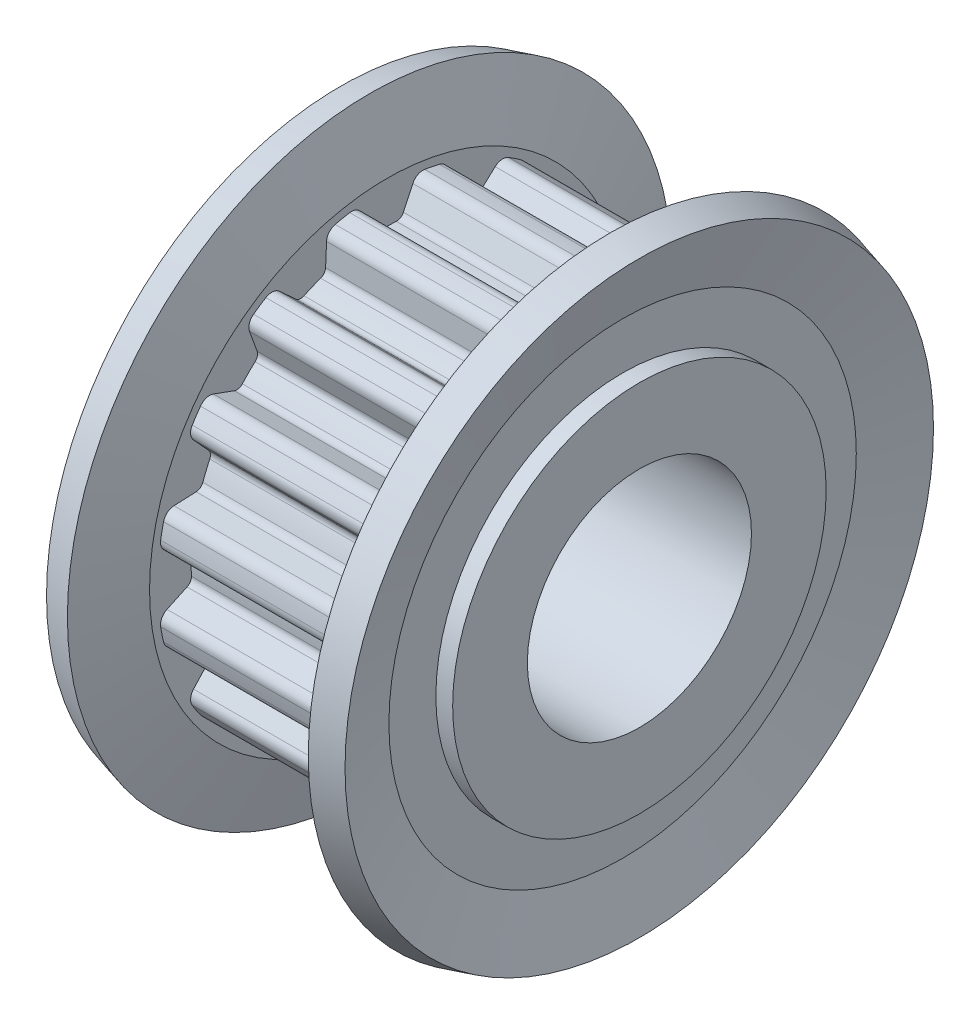
from build123d import *

# Parameters (mm, degrees)
SKETCH_2_W          = 64
SKETCH_2_H          = 64
CUT_EXTRUDE_1_DEPTH = 11


with BuildPart() as part:
    # 草图1 → 旋转1 (revolve)
    with BuildSketch(Plane.XY, mode=Mode.PRIVATE) as revolve_1_sk:
        Polygon((0, 9.8), (0, 6.2), (0.2, 6), (16, 6), (16, 10), (15.1, 10), (15.1, 12.513835473), (15.991930053, 15.754514664), (14.449291918, 16.179093968), (13.5, 12.73), (2.5, 12.73), (1.550708082, 16.179093968), (0.008069947, 15.754514664), (0.9, 12.513835473), (0.9, 10), (0.2, 10), align=None)
    revolve(revolve_1_sk.sketch.rotate(Axis((28, 0, 0), (-1, 0, 0)), 270), axis=Axis((28, 0, 0), (-1, 0, 0)))

    # 草图2 → 切除-拉伸1 (cut)
    with BuildSketch(Plane(origin=(2.5, 0, 0), x_dir=(0, 0, -1), z_dir=(1, 0, 0))):
        Rectangle(SKETCH_2_W, SKETCH_2_H)
        with BuildLine():
            Line((-11.421675295, -3.251314352), (-10.234355553, -3.303153851))
            ThreePointArc((-10.234355553, -3.303153851), (-10.014882256, -3.380486909), (-9.875590343, -3.566891557))
            ThreePointArc((-9.875590343, -3.566891557), (-9.700735091, -4.01817604), (-9.505270107, -4.460923692))
            ThreePointArc((-9.505270107, -4.460923692), (-9.471956373, -4.691225939), (-9.5724647, -4.901099725))
            Line((-9.5724647, -4.901099725), (-10.37537048, -5.777317628))
            ThreePointArc((-10.37537048, -5.777317628), (-10.530438739, -6.127247702), (-10.442388892, -6.499731859))
            ThreePointArc((-10.442388892, -6.499731859), (-10.336079998, -6.667492053), (-10.227076231, -6.833513866))
            ThreePointArc((-10.227076231, -6.833513866), (-10.115406006, -6.997754021), (-10.001098443, -7.160169686))
            ThreePointArc((-10.001098443, -7.160169686), (-9.690663174, -7.38406064), (-9.308027896, -7.374708689))
            Line((-9.308027896, -7.374708689), (-8.191249371, -6.968234547))
            ThreePointArc((-8.191249371, -6.968234547), (-7.958888404, -6.955692181), (-7.758865485, -7.074602913))
            ThreePointArc((-7.758865485, -7.074602913), (-7.424621202, -7.424621202), (-7.074602913, -7.758865485))
            ThreePointArc((-7.074602913, -7.758865485), (-6.955692181, -7.958888404), (-6.968234547, -8.191249371))
            Line((-6.968234547, -8.191249371), (-7.374708689, -9.308027896))
            ThreePointArc((-7.374708689, -9.308027896), (-7.384060643, -9.690663165), (-7.160169702, -10.001098431))
            ThreePointArc((-7.160169702, -10.001098431), (-6.997754029, -10.115406), (-6.833513866, -10.227076231))
            ThreePointArc((-6.833513866, -10.227076231), (-6.667492045, -10.336080003), (-6.499731842, -10.442388902))
            ThreePointArc((-6.499731842, -10.442388902), (-6.127247693, -10.530438738), (-5.777317628, -10.37537048))
            Line((-5.777317628, -10.37537048), (-4.901099725, -9.5724647))
            ThreePointArc((-4.901099725, -9.5724647), (-4.691225939, -9.471956373), (-4.460923692, -9.505270107))
            ThreePointArc((-4.460923692, -9.505270107), (-4.01817604, -9.700735091), (-3.566891557, -9.875590343))
            ThreePointArc((-3.566891557, -9.875590343), (-3.380486909, -10.014882256), (-3.303153851, -10.234355553))
            Line((-3.303153851, -10.234355553), (-3.251314352, -11.421675295))
            ThreePointArc((-3.251314352, -11.421675295), (-3.113526253, -11.778763026), (-2.787879562, -11.979888461))
            ThreePointArc((-2.787879562, -11.979888461), (-2.594083433, -12.023341097), (-2.399610961, -12.063658949))
            ThreePointArc((-2.399610961, -12.063658949), (-2.20451286, -12.100831502), (-2.008839989, -12.134849068))
            ThreePointArc((-2.008839989, -12.134849068), (-1.631014293, -12.073652996), (-1.367063122, -11.796476168))
            Line((-1.367063122, -11.796476168), (-0.864802075, -10.719373878))
            ThreePointArc((-0.864802075, -10.719373878), (-0.709366852, -10.54620107), (-0.483846705, -10.488846093))
            ThreePointArc((-0.483846705, -10.488846093), (0, -10.5), (0.483846705, -10.488846093))
            ThreePointArc((0.483846705, -10.488846093), (0.709366852, -10.54620107), (0.864802075, -10.719373878))
            Line((0.864802075, -10.719373878), (1.367063122, -11.796476168))
            ThreePointArc((1.367063122, -11.796476168), (1.631014267, -12.073652983), (2.00883993, -12.134849078))
            ThreePointArc((2.00883993, -12.134849078), (2.204512831, -12.100831508), (2.399610961, -12.063658949))
            ThreePointArc((2.399610961, -12.063658949), (2.594083423, -12.023341099), (2.787879543, -11.979888466))
            ThreePointArc((2.787879543, -11.979888466), (3.113526247, -11.778763034), (3.251314352, -11.421675295))
            Line((3.251314352, -11.421675295), (3.303153851, -10.234355553))
            ThreePointArc((3.303153851, -10.234355553), (3.380486909, -10.014882256), (3.566891557, -9.875590343))
            ThreePointArc((3.566891557, -9.875590343), (4.01817604, -9.700735091), (4.460923692, -9.505270107))
            ThreePointArc((4.460923692, -9.505270107), (4.691225939, -9.471956373), (4.901099725, -9.5724647))
            Line((4.901099725, -9.5724647), (5.777317628, -10.37537048))
            ThreePointArc((5.777317628, -10.37537048), (6.127247683, -10.530438737), (6.499731825, -10.442388912))
            ThreePointArc((6.499731825, -10.442388912), (6.667492036, -10.336080009), (6.833513866, -10.227076231))
            ThreePointArc((6.833513866, -10.227076231), (6.997754021, -10.115406006), (7.160169686, -10.001098443))
            ThreePointArc((7.160169686, -10.001098443), (7.38406064, -9.690663174), (7.374708689, -9.308027896))
            Line((7.374708689, -9.308027896), (6.968234547, -8.191249371))
            ThreePointArc((6.968234547, -8.191249371), (6.955692181, -7.958888404), (7.074602913, -7.758865485))
            ThreePointArc((7.074602913, -7.758865485), (7.424621202, -7.424621202), (7.758865485, -7.074602913))
            ThreePointArc((7.758865485, -7.074602913), (7.958888404, -6.955692181), (8.191249371, -6.968234547))
            Line((8.191249371, -6.968234547), (9.308027896, -7.374708689))
            ThreePointArc((9.308027896, -7.374708689), (9.690663165, -7.384060643), (10.001098431, -7.160169702))
            ThreePointArc((10.001098431, -7.160169702), (10.115406, -6.997754029), (10.227076231, -6.833513866))
            ThreePointArc((10.227076231, -6.833513866), (10.336080003, -6.667492045), (10.442388902, -6.499731842))
            ThreePointArc((10.442388902, -6.499731842), (10.530438738, -6.127247693), (10.37537048, -5.777317628))
            Line((10.37537048, -5.777317628), (9.5724647, -4.901099725))
            ThreePointArc((9.5724647, -4.901099725), (9.471956373, -4.691225939), (9.505270107, -4.460923692))
            ThreePointArc((9.505270107, -4.460923692), (9.700735091, -4.01817604), (9.875590343, -3.566891557))
            ThreePointArc((9.875590343, -3.566891557), (10.014882256, -3.380486909), (10.234355553, -3.303153851))
            Line((10.234355553, -3.303153851), (11.421675295, -3.251314352))
            ThreePointArc((11.421675295, -3.251314352), (11.778763026, -3.113526253), (11.979888461, -2.787879562))
            ThreePointArc((11.979888461, -2.787879562), (12.023341097, -2.594083433), (12.063658949, -2.399610961))
            ThreePointArc((12.063658949, -2.399610961), (12.100831502, -2.20451286), (12.134849068, -2.008839989))
            ThreePointArc((12.134849068, -2.008839989), (12.073652996, -1.631014293), (11.796476168, -1.367063122))
            Line((11.796476168, -1.367063122), (10.719373878, -0.864802075))
            ThreePointArc((10.719373878, -0.864802075), (10.54620107, -0.709366852), (10.488846093, -0.483846705))
            ThreePointArc((10.488846093, -0.483846705), (10.5, 0), (10.488846093, 0.483846705))
            ThreePointArc((10.488846093, 0.483846705), (10.54620107, 0.709366852), (10.719373878, 0.864802075))
            Line((10.719373878, 0.864802075), (11.796476168, 1.367063122))
            ThreePointArc((11.796476168, 1.367063122), (12.073652983, 1.631014267), (12.134849078, 2.00883993))
            ThreePointArc((12.134849078, 2.00883993), (12.100831508, 2.204512831), (12.063658949, 2.399610961))
            ThreePointArc((12.063658949, 2.399610961), (12.023341099, 2.594083423), (11.979888466, 2.787879543))
            ThreePointArc((11.979888466, 2.787879543), (11.778763034, 3.113526247), (11.421675295, 3.251314352))
            Line((11.421675295, 3.251314352), (10.234355553, 3.303153851))
            ThreePointArc((10.234355553, 3.303153851), (10.014882256, 3.380486909), (9.875590343, 3.566891557))
            ThreePointArc((9.875590343, 3.566891557), (9.700735091, 4.01817604), (9.505270107, 4.460923692))
            ThreePointArc((9.505270107, 4.460923692), (9.471956373, 4.691225939), (9.5724647, 4.901099725))
            Line((9.5724647, 4.901099725), (10.37537048, 5.777317628))
            ThreePointArc((10.37537048, 5.777317628), (10.530438737, 6.127247683), (10.442388912, 6.499731825))
            ThreePointArc((10.442388912, 6.499731825), (10.336080009, 6.667492036), (10.227076231, 6.833513866))
            ThreePointArc((10.227076231, 6.833513866), (10.115406006, 6.997754021), (10.001098443, 7.160169686))
            ThreePointArc((10.001098443, 7.160169686), (9.690663174, 7.38406064), (9.308027896, 7.374708689))
            Line((9.308027896, 7.374708689), (8.191249371, 6.968234547))
            ThreePointArc((8.191249371, 6.968234547), (7.958888404, 6.955692181), (7.758865485, 7.074602913))
            ThreePointArc((7.758865485, 7.074602913), (7.424621202, 7.424621202), (7.074602913, 7.758865485))
            ThreePointArc((7.074602913, 7.758865485), (6.955692181, 7.958888404), (6.968234547, 8.191249371))
            Line((6.968234547, 8.191249371), (7.374708689, 9.308027896))
            ThreePointArc((7.374708689, 9.308027896), (7.384060643, 9.690663165), (7.160169702, 10.001098431))
            ThreePointArc((7.160169702, 10.001098431), (6.997754029, 10.115406), (6.833513866, 10.227076231))
            ThreePointArc((6.833513866, 10.227076231), (6.667492045, 10.336080003), (6.499731842, 10.442388902))
            ThreePointArc((6.499731842, 10.442388902), (6.127247693, 10.530438738), (5.777317628, 10.37537048))
            Line((5.777317628, 10.37537048), (4.901099725, 9.5724647))
            ThreePointArc((4.901099725, 9.5724647), (4.691225939, 9.471956373), (4.460923692, 9.505270107))
            ThreePointArc((4.460923692, 9.505270107), (4.01817604, 9.700735091), (3.566891557, 9.875590343))
            ThreePointArc((3.566891557, 9.875590343), (3.380486909, 10.014882256), (3.303153851, 10.234355553))
            Line((3.303153851, 10.234355553), (3.251314352, 11.421675295))
            ThreePointArc((3.251314352, 11.421675295), (3.113526253, 11.778763026), (2.787879562, 11.979888461))
            ThreePointArc((2.787879562, 11.979888461), (2.594083433, 12.023341097), (2.399610961, 12.063658949))
            ThreePointArc((2.399610961, 12.063658949), (2.20451286, 12.100831502), (2.008839989, 12.134849068))
            ThreePointArc((2.008839989, 12.134849068), (1.631014293, 12.073652996), (1.367063122, 11.796476168))
            Line((1.367063122, 11.796476168), (0.864802075, 10.719373878))
            ThreePointArc((0.864802075, 10.719373878), (0.709366852, 10.54620107), (0.483846705, 10.488846093))
            ThreePointArc((0.483846705, 10.488846093), (0, 10.5), (-0.483846705, 10.488846093))
            ThreePointArc((-0.483846705, 10.488846093), (-0.709366852, 10.54620107), (-0.864802075, 10.719373878))
            Line((-0.864802075, 10.719373878), (-1.367063122, 11.796476168))
            ThreePointArc((-1.367063122, 11.796476168), (-1.631014285, 12.073652992), (-2.008839969, 12.134849071))
            ThreePointArc((-2.008839969, 12.134849071), (-2.204512851, 12.100831504), (-2.399610961, 12.063658949))
            ThreePointArc((-2.399610961, 12.063658949), (-2.594083423, 12.0233411), (-2.787879543, 11.979888466))
            ThreePointArc((-2.787879543, 11.979888466), (-3.113526247, 11.778763034), (-3.251314352, 11.421675295))
            Line((-3.251314352, 11.421675295), (-3.303153851, 10.234355553))
            ThreePointArc((-3.303153851, 10.234355553), (-3.380486909, 10.014882256), (-3.566891557, 9.875590343))
            ThreePointArc((-3.566891557, 9.875590343), (-4.01817604, 9.700735091), (-4.460923692, 9.505270107))
            ThreePointArc((-4.460923692, 9.505270107), (-4.691225939, 9.471956373), (-4.901099725, 9.5724647))
            Line((-4.901099725, 9.5724647), (-5.777317628, 10.37537048))
            ThreePointArc((-5.777317628, 10.37537048), (-6.127247683, 10.530438737), (-6.499731825, 10.442388912))
            ThreePointArc((-6.499731825, 10.442388912), (-6.667492036, 10.336080009), (-6.833513866, 10.227076231))
            ThreePointArc((-6.833513866, 10.227076231), (-6.997754021, 10.115406006), (-7.160169686, 10.001098443))
            ThreePointArc((-7.160169686, 10.001098443), (-7.38406064, 9.690663175), (-7.374708689, 9.308027896))
            Line((-7.374708689, 9.308027896), (-6.968234547, 8.191249371))
            ThreePointArc((-6.968234547, 8.191249371), (-6.955692181, 7.958888404), (-7.074602913, 7.758865485))
            ThreePointArc((-7.074602913, 7.758865485), (-7.424621202, 7.424621202), (-7.758865485, 7.074602913))
            ThreePointArc((-7.758865485, 7.074602913), (-7.958888404, 6.955692181), (-8.191249371, 6.968234547))
            Line((-8.191249371, 6.968234547), (-9.308027896, 7.374708689))
            ThreePointArc((-9.308027896, 7.374708689), (-9.690663174, 7.38406064), (-10.001098443, 7.160169686))
            ThreePointArc((-10.001098443, 7.160169686), (-10.115406006, 6.997754021), (-10.227076231, 6.833513866))
            ThreePointArc((-10.227076231, 6.833513866), (-10.336080003, 6.667492045), (-10.442388902, 6.499731842))
            ThreePointArc((-10.442388902, 6.499731842), (-10.530438738, 6.127247693), (-10.37537048, 5.777317628))
            Line((-10.37537048, 5.777317628), (-9.5724647, 4.901099725))
            ThreePointArc((-9.5724647, 4.901099725), (-9.471956373, 4.691225939), (-9.505270107, 4.460923692))
            ThreePointArc((-9.505270107, 4.460923692), (-9.700735091, 4.01817604), (-9.875590343, 3.566891557))
            ThreePointArc((-9.875590343, 3.566891557), (-10.014882256, 3.380486909), (-10.234355553, 3.303153851))
            Line((-10.234355553, 3.303153851), (-11.421675295, 3.251314352))
            ThreePointArc((-11.421675295, 3.251314352), (-11.778763042, 3.113526241), (-11.97988847, 2.787879524))
            ThreePointArc((-11.97988847, 2.787879524), (-12.023341102, 2.594083413), (-12.063658949, 2.399610961))
            ThreePointArc((-12.063658949, 2.399610961), (-12.100831502, 2.20451286), (-12.134849068, 2.008839989))
            ThreePointArc((-12.134849068, 2.008839989), (-12.073652996, 1.631014293), (-11.796476168, 1.367063122))
            Line((-11.796476168, 1.367063122), (-10.719373878, 0.864802075))
            ThreePointArc((-10.719373878, 0.864802075), (-10.54620107, 0.709366852), (-10.488846093, 0.483846705))
            ThreePointArc((-10.488846093, 0.483846705), (-10.5, 0), (-10.488846093, -0.483846705))
            ThreePointArc((-10.488846093, -0.483846705), (-10.54620107, -0.709366852), (-10.719373878, -0.864802075))
            Line((-10.719373878, -0.864802075), (-11.796476168, -1.367063122))
            ThreePointArc((-11.796476168, -1.367063122), (-12.073653001, -1.631014302), (-12.134849065, -2.008840008))
            ThreePointArc((-12.134849065, -2.008840008), (-12.100831501, -2.20451287), (-12.063658949, -2.399610961))
            ThreePointArc((-12.063658949, -2.399610961), (-12.023341099, -2.594083423), (-11.979888466, -2.787879543))
            ThreePointArc((-11.979888466, -2.787879543), (-11.778763034, -3.113526247), (-11.421675295, -3.251314352))
        make_face(mode=Mode.SUBTRACT)
    extrude(amount=CUT_EXTRUDE_1_DEPTH, mode=Mode.SUBTRACT)


solid = part.part
